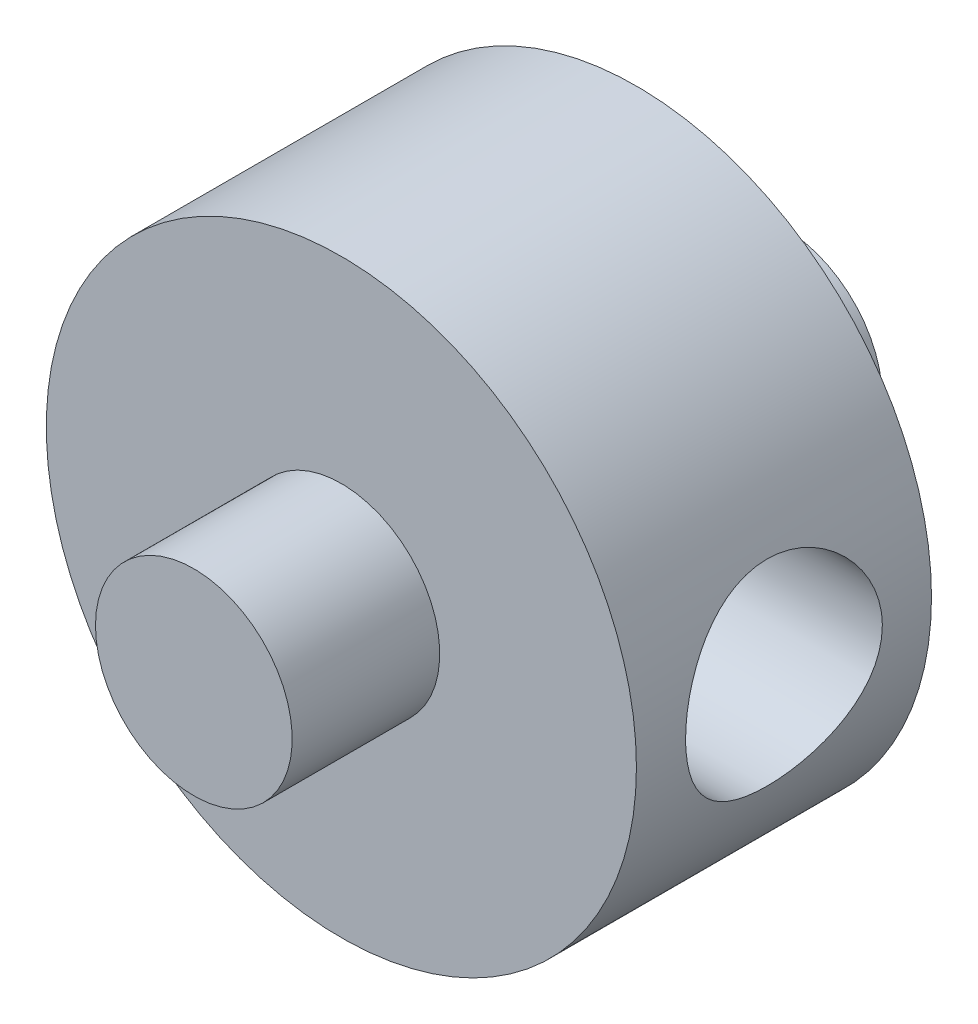
from build123d import *

# Parameters (mm, degrees)
SKETCH1_R           = 9.525
BOSS_EXTRUDE1_DEPTH = 9.525
SKETCH2_R           = 3.175
BOSS_EXTRUDE2_DEPTH = 4.7625
BOSS_EXTRUDE3_START = 4.7625
SKETCH3_R           = 3.175
BOSS_EXTRUDE3_DEPTH = 4.7625
SKETCH4_R           = 3.175
CUT_EXTRUDE1_DEPTH  = 20.636290542


with BuildPart() as part:
    # Sketch1 → Boss-Extrude1 (new body)
    with BuildSketch(Plane.XY):
        Circle(SKETCH1_R)
    extrude(amount=-BOSS_EXTRUDE1_DEPTH)

    # Sketch2 → Boss-Extrude2 (add)
    with BuildSketch(Plane.XY):
        with Locations(Location((0, 0, 0), (0, 0, 180))):
            Circle(SKETCH2_R)
    extrude(amount=BOSS_EXTRUDE2_DEPTH)

    # Sketch3 → Boss-Extrude3 (add)
    with BuildSketch(Plane(origin=(0, 0, -9.525), x_dir=(-1, 0, 0), z_dir=(0, 0, -1)).offset(BOSS_EXTRUDE3_START)):
        Circle(SKETCH3_R)
    extrude(amount=-BOSS_EXTRUDE3_DEPTH)

    # Sketch4 → Cut-Extrude1 (cut, through all)
    with BuildSketch(Plane(origin=(0, 0, 0), x_dir=(0, 0, -1), z_dir=(1, 0, 0))):
        with Locations((4.7625, 0)):
            Circle(SKETCH4_R)
    extrude(amount=CUT_EXTRUDE1_DEPTH, mode=Mode.SUBTRACT)


solid = part.part
